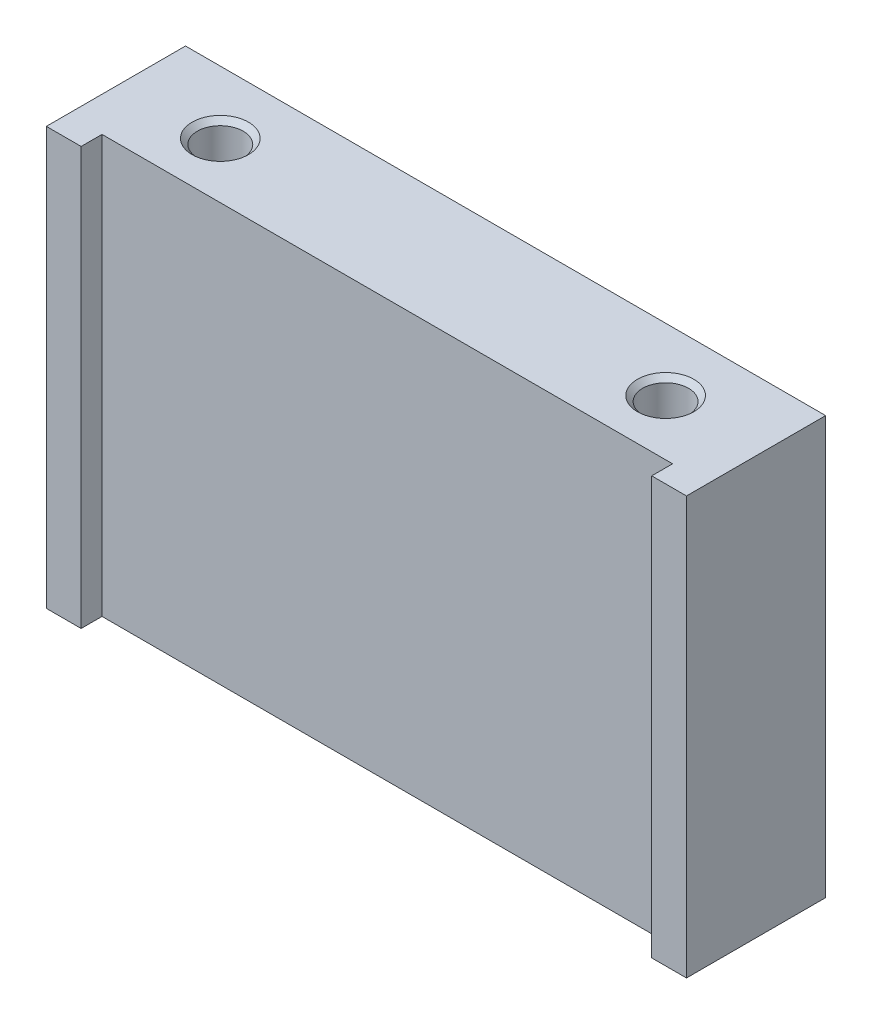
from build123d import *

# Parameters (mm, degrees)
SKETCH_1_W          = 46
SKETCH_1_H          = 30
EXTRUDE_1_DEPTH     = 10
SKETCH_2_W          = 41
SKETCH_2_H          = 30
CUT_EXTRUDE_1_DEPTH = 1.5


with BuildPart() as part:
    # 草图1 → 凸台-拉伸1 (new body)
    with BuildSketch(Plane.XY):
        Rectangle(SKETCH_1_W, SKETCH_1_H)
    extrude(amount=EXTRUDE_1_DEPTH)

    # 草图2 → 切除-拉伸1 (cut)
    with BuildSketch(Plane.XY.offset(10)):
        Rectangle(SKETCH_2_W, SKETCH_2_H)
    extrude(amount=-CUT_EXTRUDE_1_DEPTH, mode=Mode.SUBTRACT)

    # 草图3 → M4 螺纹孔1 (revolve, cut)
    with BuildSketch(Plane(origin=(16, 15, 4.5), x_dir=(0, 0, 1), z_dir=(1, 0, 0))):
        Polygon((0, 0), (0, 9.091420021), (1.65, 8.1), (1.65, 0.375), (2.025, 0), align=None)
    hole_wizard_m4_1 = revolve(axis=Axis((16, 21.35, 4.5), (0, -1, 0)), mode=Mode.SUBTRACT)

    # 镜向1: M4 螺纹孔1 across plane
    add(hole_wizard_m4_1.mirror(Plane(origin=(0, 0, 0), x_dir=(0, 0, 1), z_dir=(1, 0, 0))), mode=Mode.SUBTRACT)


solid = part.part
